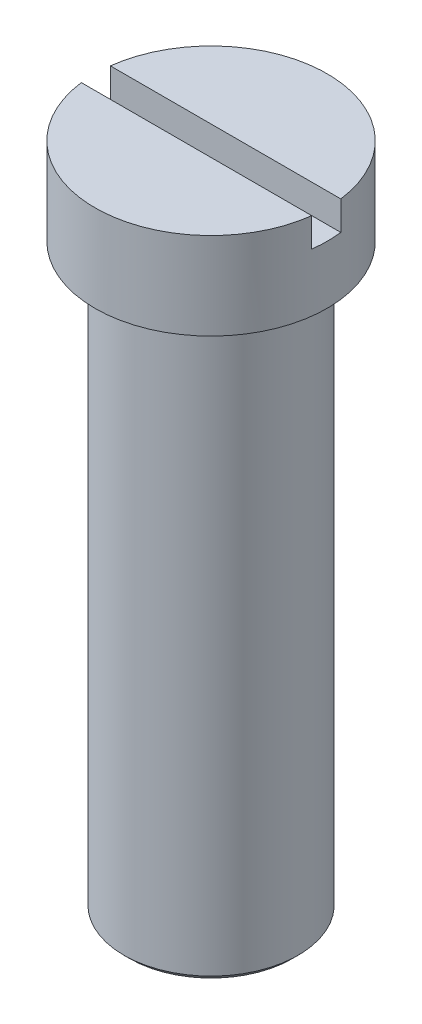
from build123d import *

# Parameters (mm, degrees)
SKETCH_1_R          = 15
EXTRUDE_1_DEPTH     = 50
SKETCH_2_R          = 20
EXTRUDE_2_DEPTH     = 15
SKETCH_3_W          = 60.184655206
SKETCH_3_H          = 5
CUT_EXTRUDE_1_DEPTH = 5
CHAMFER_1_SIZE      = 1


with BuildPart() as part:
    # 草图1 → 凸台-拉伸1 (new, symmetric)
    with BuildSketch(Plane(origin=(0, 0, 0), x_dir=(1, 0, 0), z_dir=(0, 1, 0))):
        with Locations(Location((0, 0, 0), (0, 0, 270))):
            Circle(SKETCH_1_R)
    extrude(amount=EXTRUDE_1_DEPTH, both=True)

    # 草图2 → 凸台-拉伸2 (add)
    with BuildSketch(Plane(origin=(0, 50, 0), x_dir=(1, 0, 0), z_dir=(0, 1, 0))):
        with Locations(Location((0, 0, 0), (0, 0, 270))):
            Circle(SKETCH_2_R)
    extrude(amount=EXTRUDE_2_DEPTH)

    # 草图3 → 切除-拉伸1 (cut)
    with BuildSketch(Plane(origin=(0, 65, 0), x_dir=(1, 0, 0), z_dir=(0, 1, 0))):
        Rectangle(SKETCH_3_W, SKETCH_3_H)
    extrude(amount=-CUT_EXTRUDE_1_DEPTH, mode=Mode.SUBTRACT)

    # 倒角1
    chamfer_1_edges = [part.edges().sort_by_distance(p)[0] for p in [
        (0, -50, -15),
    ]]
    chamfer(chamfer_1_edges, length=CHAMFER_1_SIZE)


solid = part.part
